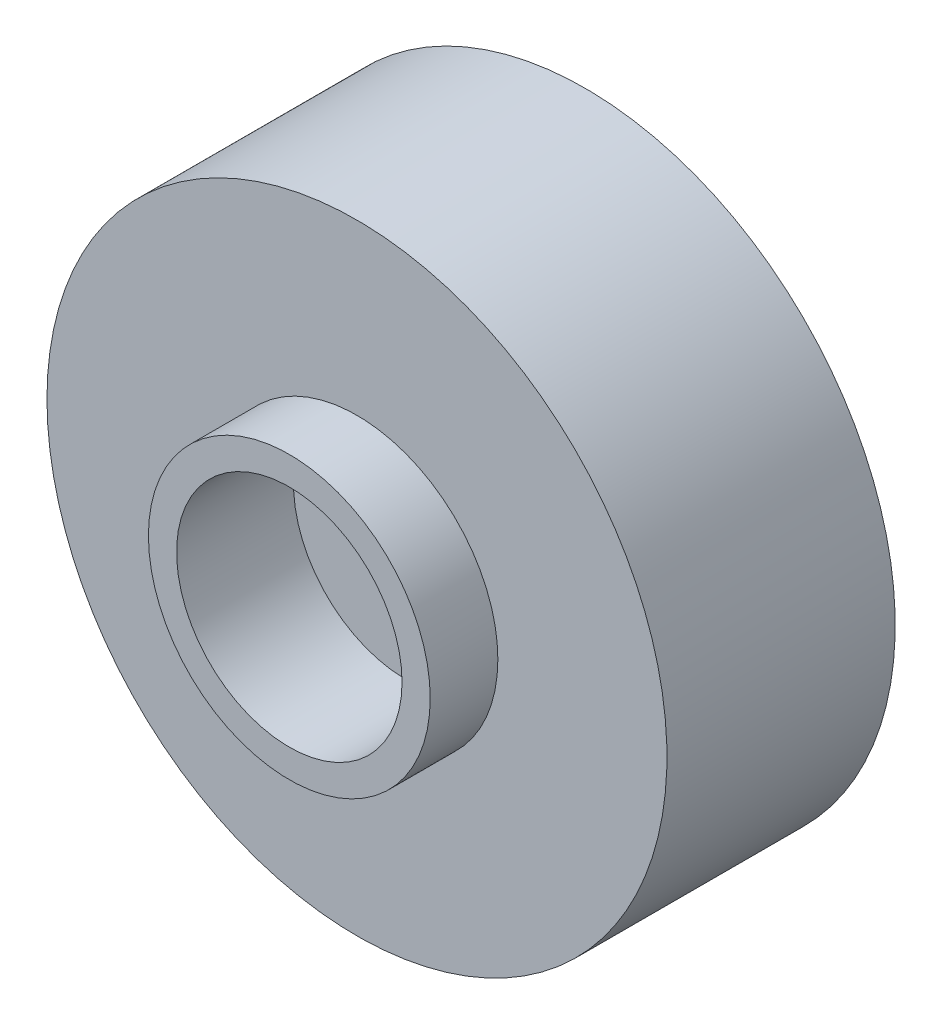
from build123d import *

# Parameters (mm, degrees)
SKETCH1_R           = 11
BOSS_EXTRUDE1_DEPTH = 10.5
SKETCH2_OUTSIDE_W   = 30.568
SKETCH2_OUTSIDE_H   = 30.568
SKETCH2_OUTSIDE_R   = 5
CUT_EXTRUDE1_DEPTH  = 2.4
SKETCH3_R           = 4
CUT_EXTRUDE2_DEPTH  = 4.15
SKETCH4_R           = 8.75
CUT_EXTRUDE3_DEPTH  = 3
CHAMFER1_SIZE       = 0.2


with BuildPart() as part:
    # Sketch1 → Boss-Extrude1 (new body)
    with BuildSketch(Plane.XY):
        with Locations(Location((0, 0, 0), (0, 0, 180))):
            Circle(SKETCH1_R)
    extrude(amount=BOSS_EXTRUDE1_DEPTH)

    # Sketch2 outside → Cut-Extrude1 (cut)
    with BuildSketch(Plane.XY.offset(10.5)):
        Rectangle(SKETCH2_OUTSIDE_W, SKETCH2_OUTSIDE_H)
        Circle(SKETCH2_OUTSIDE_R, mode=Mode.SUBTRACT)
    extrude(amount=-CUT_EXTRUDE1_DEPTH, mode=Mode.SUBTRACT)

    # Sketch3 → Cut-Extrude2 (cut)
    with BuildSketch(Plane.XY.offset(10.5)):
        Circle(SKETCH3_R)
    extrude(amount=-CUT_EXTRUDE2_DEPTH, mode=Mode.SUBTRACT)

    # Sketch4 → Cut-Extrude3 (cut)
    with BuildSketch(Plane(origin=(0, 0, 0), x_dir=(-1, 0, 0), z_dir=(0, 0, -1))):
        Circle(SKETCH4_R)
    extrude(amount=-CUT_EXTRUDE3_DEPTH, mode=Mode.SUBTRACT)

    # Chamfer1
    chamfer1_edges = [part.edges().sort_by_distance(p)[0] for p in [
        (8.75, 0, 0),
    ]]
    chamfer(chamfer1_edges, length=CHAMFER1_SIZE)


solid = part.part
